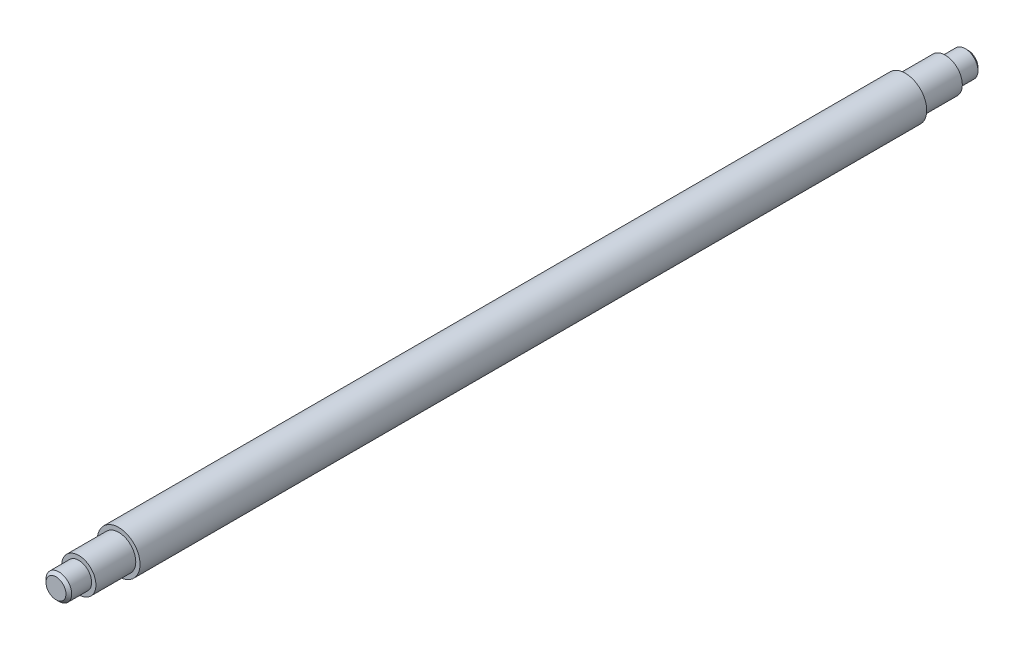
from build123d import *

# Parameters (mm, degrees)
SKETCH_1_R      = 4.5
EXTRUDE_1_DEPTH = 8
SKETCH_2_R      = 6
EXTRUDE_2_DEPTH = 14
SKETCH_3_R      = 7.5
EXTRUDE_3_DEPTH = 276
SKETCH_4_R      = 6
EXTRUDE_4_DEPTH = 14
SKETCH_5_R      = 4.5
EXTRUDE_5_DEPTH = 8
CHAMFER_1_SIZE  = 1


with BuildPart() as part:
    # 草图1 → 凸台-拉伸1 (new body)
    with BuildSketch(Plane.XY):
        Circle(SKETCH_1_R)
    extrude(amount=EXTRUDE_1_DEPTH)

    # 草图2 → 凸台-拉伸2 (add)
    with BuildSketch(Plane.XY.offset(8)):
        Circle(SKETCH_2_R)
    extrude(amount=EXTRUDE_2_DEPTH)

    # 草图3 → 凸台-拉伸3 (add)
    with BuildSketch(Plane.XY.offset(22)):
        Circle(SKETCH_3_R)
    extrude(amount=EXTRUDE_3_DEPTH)

    # 草图4 → 凸台-拉伸4 (add)
    with BuildSketch(Plane.XY.offset(298)):
        Circle(SKETCH_4_R)
    extrude(amount=EXTRUDE_4_DEPTH)

    # 草图5 → 凸台-拉伸5 (add)
    with BuildSketch(Plane.XY.offset(312)):
        Circle(SKETCH_5_R)
    extrude(amount=EXTRUDE_5_DEPTH)

    # 倒角1
    chamfer_1_edges = [part.edges().sort_by_distance(p)[0] for p in [
        (-4.5, 0, 0),
        (-4.5, 0, 320),
    ]]
    chamfer(chamfer_1_edges, length=CHAMFER_1_SIZE)


solid = part.part
